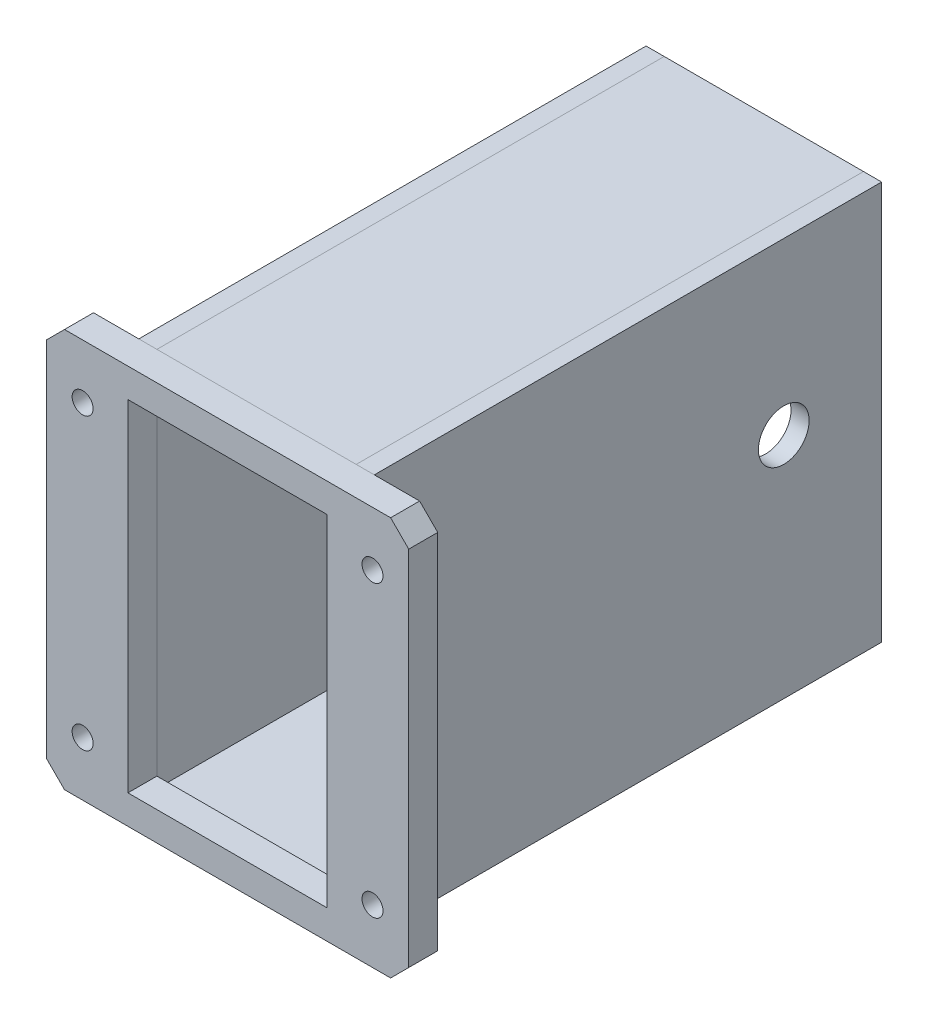
SolidWorks part; units mm, degrees
material "Q235"
ref_plane "Front Plane" through (0, 0, 0) normal (0, 0, 1) x (1, 0, 0)
ref_plane "Top Plane" through (0, 0, 0) normal (0, 1, 0) x (1, 0, 0)
ref_plane "Right Plane" through (0, 0, 0) normal (1, 0, 0) x (0, 0, -1)
sketch "Sketch1" plane through (0, 0, 0) normal (0, 0, 1) x (1, 0, 0)
  line L1 (-50, 55) -> (50, 55)
  line L2 (-50, 55) -> (-50, -55)
  line L3 (-50, -55) -> (50, -55)
  line L4 (50, 55) -> (50, -55)
  line L5 (-50, 55) -> (50, -55) construction
  line L6 (-50, -55) -> (50, 55) construction
  point P0 (0, 0)
  dimension "D1" = 110
  dimension "D2" = 100
extrude "Boss-Extrude1" add sketch "Sketch1" along normal blind 8
sketch "Sketch2" plane through (0, 0, 8) normal (0, 0, 1) x (1, 0, 0)
  line L0 (50, 55) -> (-50, 55) construction
  line L1 (-27.5, 47) -> (27.5, 47)
  line L2 (-27.5, 47) -> (-27.5, -47)
  line L3 (-27.5, -47) -> (27.5, -47)
  line L4 (27.5, 47) -> (27.5, -47)
  line L5 (-27.5, 47) -> (27.5, -47) construction
  line L6 (-27.5, -47) -> (27.5, 47) construction
  point P0 (0, 0)
  dimension "D1" = 8
  dimension "D2" = 55
extrude "Cut-Extrude1" cut sketch "Sketch2" against normal blind 8
sketch "Sketch3" plane through (0, 0, 0) normal (0, 0, -1) x (-1, 0, 0)
  line L0 (-27.5, -47) -> (-27.5, 47) construction
  line L10 (-50, 55) -> (50, 55) construction
  line L11 (-32.5, 55) -> (-27.5, 55)
  line L12 (-32.5, 55) -> (-32.5, -55)
  line L13 (-32.5, -55) -> (-27.5, -55)
  line L14 (-27.5, 55) -> (-27.5, -55)
  line L15 (50, -55) -> (-50, -55) construction
  line L17 (0, 0) -> (0, 29.7546) construction
  line L18 (27.5, 55) -> (27.5, -55)
  line L19 (32.5, -55) -> (27.5, -55)
  line L20 (32.5, 55) -> (32.5, -55)
  line L21 (32.5, 55) -> (27.5, 55)
  dimension "D1" = 5
  dimension "D2" = 0
extrude "Boss-Extrude2" add sketch "Sketch3" along normal blind 140 separate body
sketch "Sketch4" plane through (0, 0, 0) normal (0, 0, -1) x (-1, 0, 0)
  line L5 (-27.5, 50) -> (27.5, 50)
  line L6 (-27.5, 50) -> (-27.5, 55)
  line L7 (-27.5, 55) -> (27.5, 55)
  line L8 (27.5, 50) -> (27.5, 55)
  line L9 (-27.5, 0) -> (-10.4049, 0) construction
  line L10 (-27.5, -55) -> (-27.5, 55) construction
  line L11 (27.5, -50) -> (27.5, -55)
  line L12 (-27.5, -55) -> (27.5, -55)
  line L13 (-27.5, -50) -> (-27.5, -55)
  line L14 (-27.5, -50) -> (27.5, -50)
  line L15 (-50, 55) -> (50, 55) construction
  line L16 (-27.5, -55) -> (-27.5, 55) construction
  line L17 (-27.5, -55) -> (-27.5, 55) construction
  line L18 (27.5, 55) -> (27.5, -55) construction
  dimension "D1" = 5
extrude "Boss-Extrude3" add sketch "Sketch4" along normal blind 140 separate body
chamfer "Chamfer1" distance 5 angle 45 4 edges at (50, -55, 4) (-50, -55, 4) (-50, 55, 4) (50, 55, 4)
hole_wizard "M5 Clearance Hole1" positions "Sketch5" profile "Sketch6" hole size "M5" standard "GB" end condition through all
sketch "Sketch5" plane through (0, 0, 8) normal (0, 0, 1) x (1, 0, 0)
  line L0 (0, 55) -> (0, 0) construction
  line L1 (45, 55) -> (-45, 55) construction
  line L3 (27.5, 0) -> (50, 0) construction
  line L4 (27.5, -47) -> (27.5, 47) construction
  line L5 (50, -50) -> (50, 50) construction
  point P0 (-40, 40)
  point P2 (-40, -40)
  point P10 (40, -40)
  point P11 (40, 40)
  dimension "D1" = 80
  dimension "D2" = 80
sketch "Sketch6" plane through (-40, 40, 8) normal (1, 0, 0) x (0, -1, 0)
  line L0 (0, 0) -> (0, 148)
  line L1 (0, 148) -> (2.9, 148)
  line L2 (2.9, 148) -> (2.9, 0)
  line L5 (2.9, 0) -> (0, 0)
  line L11 (0, -6.35) -> (0, 107.95) construction
  dimension "通孔孔直径" = 5.8
  dimension "通孔孔深度" = 148
sketch "Sketch7" plane through (32.5, 0, 0) normal (1, 0, 0) x (0, 0, -1)
  line L0 (140, -55) -> (0, -55) construction
  line L2 (0, -50) -> (0, 50) construction
  circle A0 centre (113, 8) radius 7
  dimension "D1" = 14
  dimension "D2" = 63
  dimension "D3" = 113
extrude "Cut-Extrude2" cut sketch "Sketch7" against normal through all
